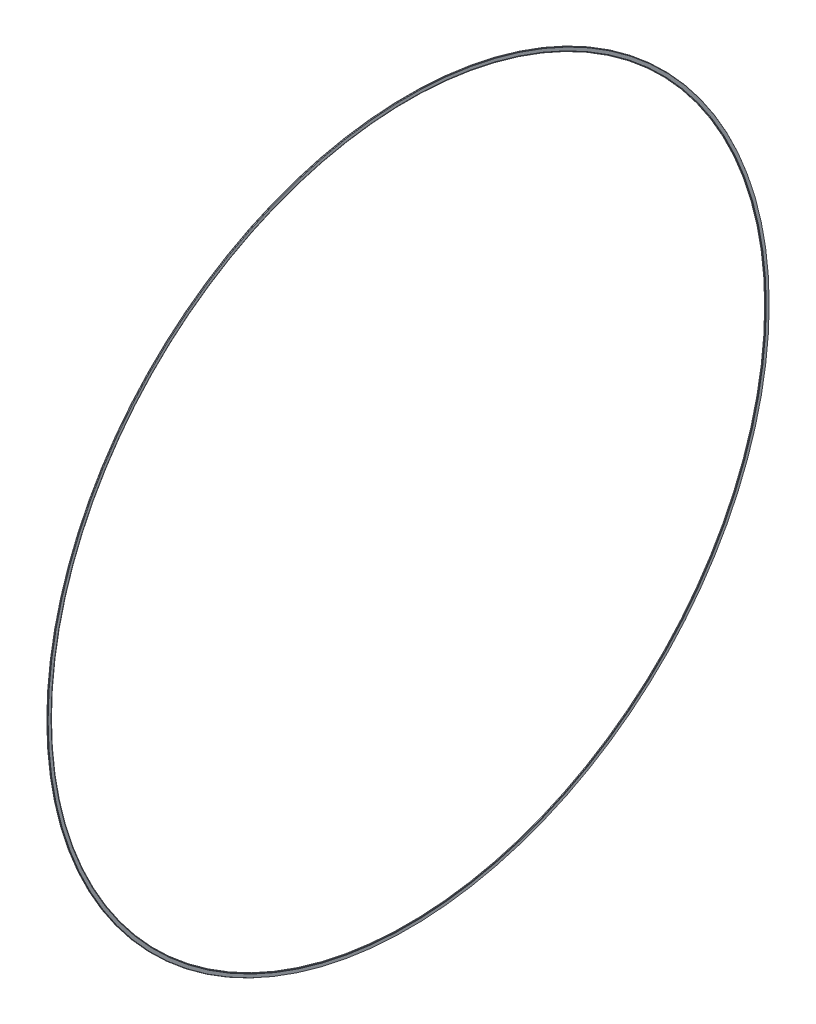
from build123d import *


with BuildPart() as part:
    # 草图1 → 旋转1 (revolve)
    with BuildSketch(Plane.XY, mode=Mode.PRIVATE) as revolve_1_sk:
        with BuildLine():
            Line((0, 148.3), (0.15, 148.3))
            ThreePointArc((0.15, 148.3), (0.260426662, 148.203354538), (0.4, 148.158037035))
            Line((0.4, 148.158037035), (0.4, 146.935990161))
            Line((0.4, 146.935990161), (0.312098656, 146.7))
            Line((0.312098656, 146.7), (0, 146.7))
            Line((0, 146.7), (0, 148.3))
        make_face()
    revolve(revolve_1_sk.sketch.rotate(Axis((0, 0, 0), (1, 0, 0)), 90), axis=Axis((0, 0, 0), (1, 0, 0)))


solid = part.part
